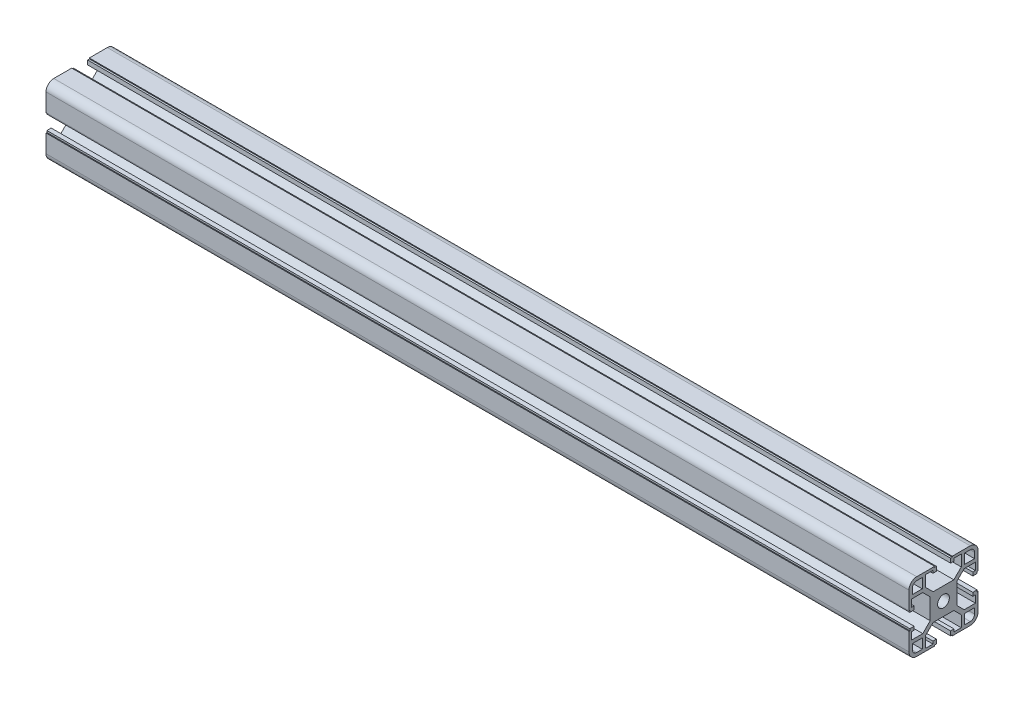
SolidWorks part; units mm, degrees
ref_plane "Front Plane" through (0, 0, 0) normal (0, 0, 1) x (1, 0, 0)
ref_plane "Top Plane" through (0, 0, 0) normal (0, 1, 0) x (1, 0, 0)
ref_plane "Right Plane" through (0, 0, 0) normal (1, 0, 0) x (0, 0, -1)
sketch "草图1" plane through (0, 0, 0) normal (0, 0, 1) x (1, 0, 0)
  line L0 (0, 0) -> (500, 0)
  dimension "D1" = 500
other "Aluminum profile 40 X 40B X R4.5(1)"
ref_plane "Plane1" through (0, 0, 0) normal (1, 0, 0) x (0, 1, 0)
sketch "Sketch1" plane through (0, 0, 0) normal (1, 0, 0) x (0, 1, 0)
  line L0 (-5.1, 20) -> (-5.1, 19.5)
  line L1 (-5.1, 19.5) -> (-4.1, 19.5)
  line L2 (-4.1, 19.5) -> (-4.1, 17)
  line L3 (-6.1, 18.5) -> (-10.3, 18.5)
  line L4 (-15.5, -20) -> (-5.1, -20)
  line L5 (-20, -15.5) -> (-20, -5.1)
  line L6 (15.5, 20) -> (5.1, 20)
  line L7 (20, 15.5) -> (20, 5.1)
  line L8 (0, 14.8756) -> (0, 0) construction
  line L9 (0, 0) -> (14.1675, 0) construction
  line L10 (-10.3, 18.5) -> (-10.3, 12)
  line L11 (-10.3, 12) -> (-6, 7.7)
  line L12 (-6, 7.7) -> (6, 7.7)
  line L13 (10.3, 12) -> (6, 7.7)
  line L14 (10.3, 18.5) -> (10.3, 12)
  line L15 (6.1, 18.5) -> (10.3, 18.5)
  line L16 (4.1, 19.5) -> (4.1, 17)
  line L17 (5.1, 19.5) -> (4.1, 19.5)
  line L18 (5.1, 20) -> (5.1, 19.5)
  line L19 (-5.1, 20) -> (-15.5, 20)
  line L20 (20, 5.1) -> (19.5, 5.1)
  line L21 (12.3, 18) -> (15.5, 18)
  line L22 (12.3, 18) -> (12.3, 12.3)
  line L23 (12.3, 12.3) -> (18, 12.3)
  line L24 (18, 15.5) -> (18, 12.3)
  line L25 (19.5, 5.1) -> (19.5, 4.1)
  line L26 (19.5, 4.1) -> (17, 4.1)
  line L27 (17, 6.1) -> (17, 4.1)
  line L28 (18.5, 6.1) -> (17, 6.1)
  line L29 (18.5, 6.1) -> (18.5, 10.3)
  line L30 (18.5, 10.3) -> (12, 10.3)
  line L31 (12, 10.3) -> (7.7, 6)
  line L32 (7.7, 6) -> (7.7, -6)
  line L33 (12, -10.3) -> (7.7, -6)
  line L34 (18.5, -10.3) -> (12, -10.3)
  line L35 (18.5, -6.1) -> (18.5, -10.3)
  line L36 (18.5, -6.1) -> (17, -6.1)
  line L37 (17, -4.1) -> (17, -6.1)
  line L38 (19.5, -4.1) -> (17, -4.1)
  line L39 (19.5, -5.1) -> (19.5, -4.1)
  line L40 (20, -5.1) -> (19.5, -5.1)
  line L41 (5.1, -20) -> (5.1, -19.5)
  line L42 (5.1, -19.5) -> (4.1, -19.5)
  line L43 (4.1, -19.5) -> (4.1, -17)
  line L44 (6.1, -17) -> (4.1, -17)
  line L45 (6.1, -18.5) -> (6.1, -17)
  line L46 (6.1, -18.5) -> (10.3, -18.5)
  line L47 (10.3, -18.5) -> (10.3, -12)
  line L48 (10.3, -12) -> (6, -7.7)
  line L49 (6, -7.7) -> (-6, -7.7)
  line L50 (-10.3, -12) -> (-6, -7.7)
  line L51 (-10.3, -18.5) -> (-10.3, -12)
  line L52 (-6.1, -18.5) -> (-10.3, -18.5)
  line L53 (-6.1, -18.5) -> (-6.1, -17)
  line L54 (-4.1, -17) -> (-6.1, -17)
  line L55 (-4.1, -19.5) -> (-4.1, -17)
  line L56 (-5.1, -19.5) -> (-4.1, -19.5)
  line L57 (-5.1, -20) -> (-5.1, -19.5)
  line L58 (-20, -5.1) -> (-19.5, -5.1)
  line L59 (5.1, -20) -> (15.5, -20)
  line L60 (-20, 5.1) -> (-20, 15.5)
  line L61 (-19.5, -5.1) -> (-19.5, -4.1)
  line L62 (-6.1, 18.5) -> (-6.1, 17)
  line L63 (-6.1, 17) -> (-4.1, 17)
  line L64 (6.1, 18.5) -> (6.1, 17)
  line L65 (4.1, 17) -> (6.1, 17)
  line L66 (-19.5, -4.1) -> (-17, -4.1)
  line L67 (-15.5, 18) -> (-12.3, 18)
  line L68 (-18, 15.5) -> (-18, 12.3)
  line L69 (-18, 12.3) -> (-12.3, 12.3)
  line L70 (-12.3, 18) -> (-12.3, 12.3)
  line L71 (-17, -6.1) -> (-17, -4.1)
  line L72 (-18.5, -6.1) -> (-17, -6.1)
  line L73 (-18.5, -6.1) -> (-18.5, -10.3)
  line L74 (-18.5, -10.3) -> (-12, -10.3)
  line L75 (-12, -10.3) -> (-7.7, -6)
  line L76 (-7.7, -6) -> (-7.7, 6)
  line L77 (-12, 10.3) -> (-7.7, 6)
  line L78 (-18.5, 10.3) -> (-12, 10.3)
  line L79 (-18.5, 6.1) -> (-18.5, 10.3)
  line L80 (-18.5, 6.1) -> (-17, 6.1)
  line L81 (-17, 4.1) -> (-17, 6.1)
  line L82 (-19.5, 4.1) -> (-17, 4.1)
  line L83 (-19.5, 5.1) -> (-19.5, 4.1)
  line L84 (-20, 5.1) -> (-19.5, 5.1)
  line L85 (20, -5.1) -> (20, -15.5)
  line L87 (-18, -12.3) -> (-12.3, -12.3)
  line L88 (-18, -12.3) -> (-18, -15.5)
  line L89 (-15.5, -18) -> (-12.3, -18)
  line L90 (-12.3, -12.3) -> (-12.3, -18)
  line L91 (12.3, -12.3) -> (18, -12.3)
  line L92 (12.3, -12.3) -> (12.3, -18)
  line L93 (12.3, -18) -> (15.5, -18)
  line L94 (18, -12.3) -> (18, -15.5)
  circle A0 centre (0, 0) radius 3.4
  arc A1 (-20, 15.5) -> (-15.5, 20) centre (-15.5, 15.5) cw
  arc A2 (20, 15.5) -> (15.5, 20) centre (15.5, 15.5) ccw
  arc A3 (-15.5, -20) -> (-20, -15.5) centre (-15.5, -15.5) cw
  arc A4 (15.5, -20) -> (20, -15.5) centre (15.5, -15.5) ccw
  arc A5 (-15.5, 18) -> (-18, 15.5) centre (-15.5, 15.5) ccw
  arc A6 (18, 15.5) -> (15.5, 18) centre (15.5, 15.5) ccw
  arc A7 (18, -15.5) -> (15.5, -18) centre (15.5, -15.5) cw
  arc A8 (-18, -15.5) -> (-15.5, -18) centre (-15.5, -15.5) ccw
  point P2 (0, 10)
  point P4 (0, 0)
  point P5 (-20, -20)
  point P6 (20, -20)
  point P7 (20, 20)
  point P8 (-20, 20)
  point P36 (-20, 20)
  point P39 (20, 20)
  point P121 (0, 0)
  dimension "D1" = 20.6
  dimension "D2" = 40
  dimension "D3" = 8.2
  dimension "D4" = 10.2
  dimension "D5" = 12.3
  dimension "D6" = 6.8
  dimension "D7" = 4.5
  dimension "D8" = 45
  dimension "D12" = 2
  dimension "D13" = 5.7
  dimension "D14" = 2
  dimension "D18" = 2.5
  dimension "D19" = 2.5
  dimension "D15" = 2.5
  dimension "D9" = 0.5
  dimension "D10" = 1.5
  dimension "D11" = 12
  dimension "D16" = 3
  dimension "D17" = 2
  dimension "D20" = 2
  dimension "D21" = 2
